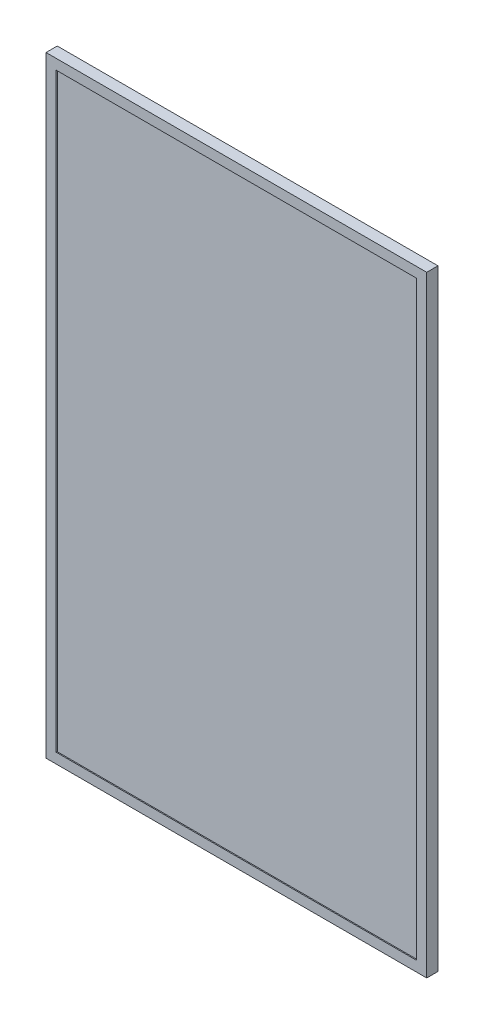
from build123d import *

# Parameters (mm, degrees)
SKETCH_1_W      = 745
SKETCH_1_H      = 1196
EXTRUDE_1_DEPTH = 22
SHELL_1_T       = -2
SKETCH_2_W      = 745
SKETCH_2_H      = 1196
SKETCH_2_W_2    = 705
SKETCH_2_H_2    = 1156
EXTRUDE_2_DEPTH = 2


with BuildPart() as part:
    # 草图1 → 凸台-拉伸1 (new body)
    with BuildSketch(Plane.XY):
        with Locations((372.5, 598)):
            Rectangle(SKETCH_1_W, SKETCH_1_H)
    extrude(amount=EXTRUDE_1_DEPTH)

    # 抽壳1
    shell_1_openings = [part.faces().sort_by_distance(p)[0] for p in [
        (372.5, 598, 22),
    ]]
    offset(amount=SHELL_1_T, openings=shell_1_openings, kind=Kind.INTERSECTION)

    # 草图2 → 凸台-拉伸2 (add)
    with BuildSketch(Plane.XY.offset(22)):
        with Locations((372.5, 598)):
            Rectangle(SKETCH_2_W, SKETCH_2_H)
        with Locations((372.5, 598)):
            Rectangle(SKETCH_2_W_2, SKETCH_2_H_2, mode=Mode.SUBTRACT)
    extrude(amount=-EXTRUDE_2_DEPTH)


solid = part.part
